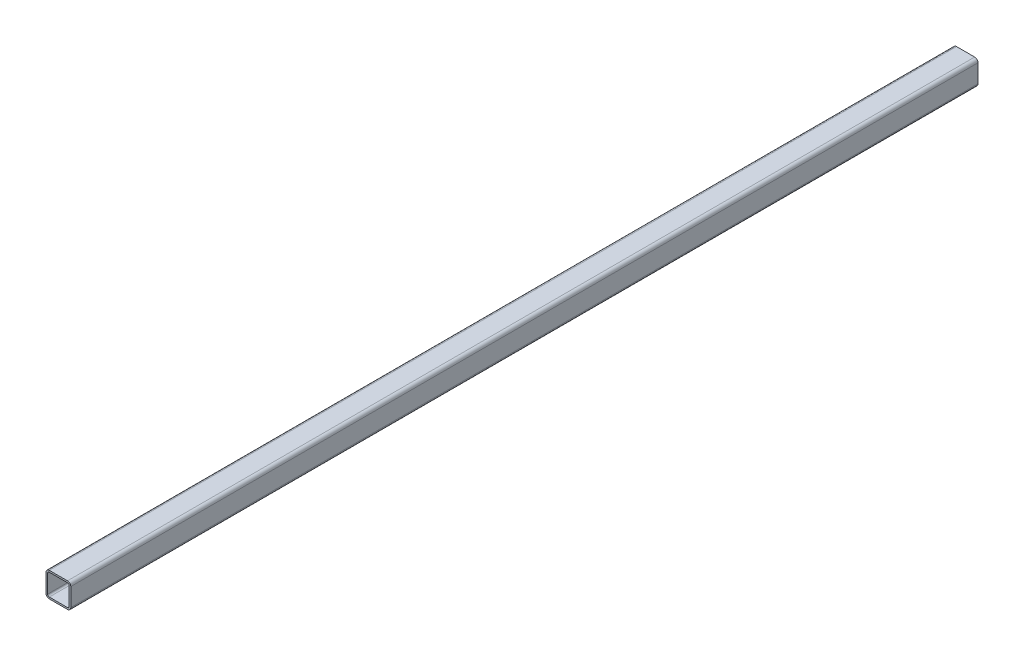
SolidWorks part; units mm, degrees
material "Q235"
ref_plane "Plane1" through (0, 0, 0) normal (0, 0, 1) x (1, 0, 0)
ref_plane "Plane2" through (0, 0, 0) normal (0, 1, 0) x (1, 0, 0)
ref_plane "Plane3" through (0, 0, 0) normal (1, 0, 0) x (0, 0, -1)
sketch "Sketch1" plane through (0, 0, 0) normal (0, 0, 1) x (1, 0, 0)
  line L0 (-11, -13) -> (11, -13)
  line L1 (-13, -11) -> (-13, 11)
  line L2 (11, 13) -> (-11, 13)
  line L3 (13, 11) -> (13, -11)
  line L4 (-11, -15) -> (11, -15)
  line L5 (-15, -11) -> (-15, 11)
  line L6 (11, 15) -> (-11, 15)
  line L7 (15, 11) -> (15, -11)
  arc A0 (15, 11) -> (11, 15) centre (11, 11) ccw
  arc A1 (11, -15) -> (15, -11) centre (11, -11) ccw
  arc A2 (-15, -11) -> (-11, -15) centre (-11, -11) ccw
  arc A3 (-11, 15) -> (-15, 11) centre (-11, 11) ccw
  arc A4 (-11, 13) -> (-13, 11) centre (-11, 11) ccw
  arc A5 (13, 11) -> (11, 13) centre (11, 11) ccw
  arc A6 (11, -13) -> (13, -11) centre (11, -11) ccw
  arc A7 (-13, -11) -> (-11, -13) centre (-11, -11) ccw
  point P0 (-15, 0)
  point P1 (15, 0)
  point P2 (0, 15)
  point P3 (0, -15)
  point P4 (0, 0)
  point P5 (-15, -15)
  point P6 (15, -15)
  point P7 (15, 15)
  point P8 (-15, 15)
  point P33 (0, 5)
  point P35 (-5, 0)
  point P36 (5, 0)
  point P37 (0, -5)
extrude "Extrude-Thin1" add sketch "Sketch1" along normal mid plane 1097.6 thin contours L6 A3 L5 A2 L4 A1 L7 A0
